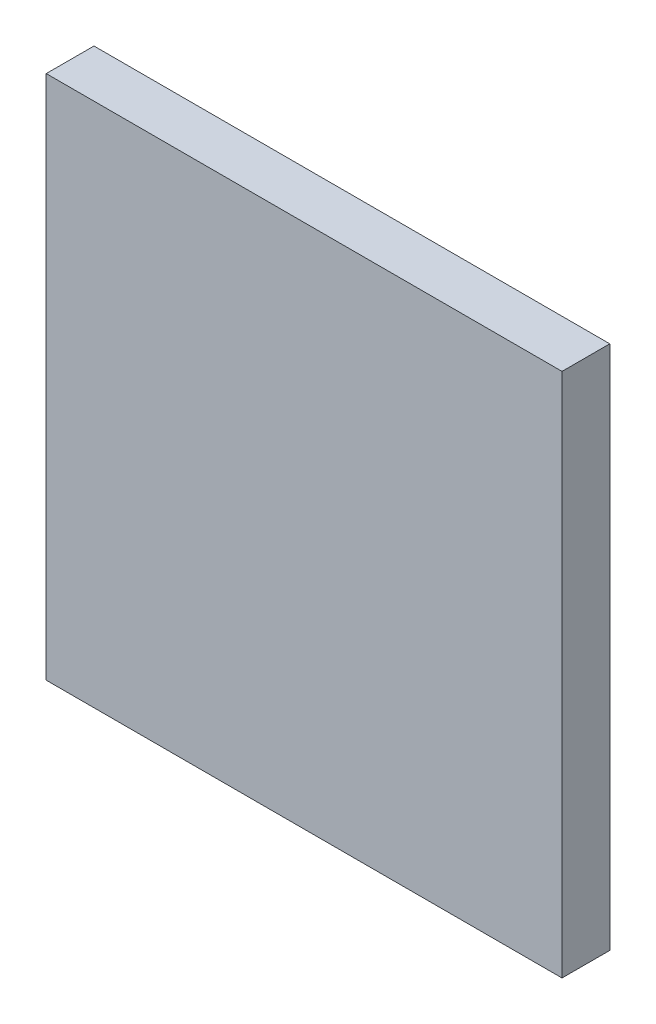
SolidWorks part; units mm, degrees
ref_plane "前视基准面" through (0, 0, 0) normal (0, 0, 1) x (1, 0, 0)
ref_plane "上视基准面" through (0, 0, 0) normal (0, 1, 0) x (1, 0, 0)
ref_plane "右视基准面" through (0, 0, 0) normal (1, 0, 0) x (0, 0, -1)
sketch "草图1" plane through (0, 0, 0) normal (0, 0, 1) x (1, 0, 0)
  line L1 (-54, -55) -> (54, -55)
  line L2 (-54, -55) -> (-54, 55)
  line L3 (-54, 55) -> (54, 55)
  line L4 (54, -55) -> (54, 55)
  line L5 (-54, -55) -> (54, 55) construction
  line L6 (-54, 55) -> (54, -55) construction
  point P0 (0, 0)
  dimension "D1" = 108
  dimension "D2" = 110
extrude "凸台-拉伸1" add sketch "草图1" along normal mid plane 10
